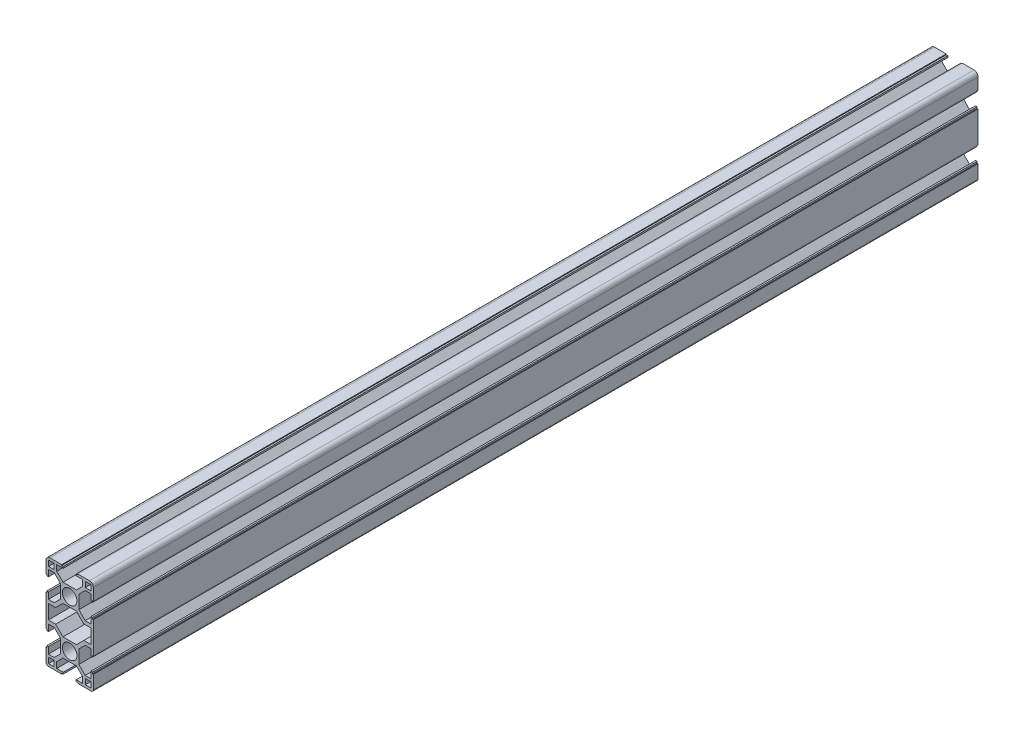
SolidWorks part; units mm, degrees
material "A6061 T6"
ref_plane "前视基准面" through (0, 0, 0) normal (0, 0, 1) x (1, 0, 0)
ref_plane "上视基准面" through (0, 0, 0) normal (0, 1, 0) x (1, 0, 0)
ref_plane "右视基准面" through (0, 0, 0) normal (1, 0, 0) x (0, 0, -1)
sketch "草图1" plane through (0, 0, 0) normal (0, 1, 0) x (1, 0, 0)
  line L0 (0, 0) -> (0, 560)
  dimension "D1" = 560
other "铝型材 30 X 60L X R2.5(1)"
ref_plane "基准面1" through (0, 0, 0) normal (0, 0, -1) x (-1, 0, 0)
sketch "Sketch1" plane through (0, 0, 0) normal (0, 0, -1) x (-1, 0, 0)
  line L0 (-5.1, 15) -> (-5.1, 14.5)
  line L1 (-5.1, 14.5) -> (-4.1, 14.5)
  line L2 (-4.1, 14.5) -> (-4.1, 13.5)
  line L3 (-4.1, 13.5) -> (-8.25, 13.5)
  line L4 (8.9, -10.45) -> (4.25, -5.8)
  line L5 (-15, -24.9) -> (-15, -5.1)
  line L6 (12.5, 15) -> (5.1, 15)
  line L7 (15, 12.5) -> (15, 5.1)
  line L8 (0, 15) -> (0, 0) construction
  line L9 (0, 0) -> (15, 0) construction
  line L10 (-8.25, 13.5) -> (-8.25, 9.8)
  line L11 (-8.25, 9.8) -> (-4.25, 5.8)
  line L12 (-4.25, 5.8) -> (4.25, 5.8)
  line L13 (8.25, 9.8) -> (4.25, 5.8)
  line L14 (8.25, 13.5) -> (8.25, 9.8)
  line L15 (4.1, 13.5) -> (8.25, 13.5)
  line L16 (4.1, 14.5) -> (4.1, 13.5)
  line L17 (5.1, 14.5) -> (4.1, 14.5)
  line L18 (5.1, 15) -> (5.1, 14.5)
  line L19 (-5.1, 15) -> (-12.5, 15)
  line L20 (15, 5.1) -> (14.5, 5.1)
  line L21 (14.5, 5.1) -> (14.5, 4.1)
  line L22 (14.5, 4.1) -> (13.5, 4.1)
  line L23 (13.5, 4.1) -> (13.5, 8.25)
  line L24 (13.5, 8.25) -> (9.8, 8.25)
  line L25 (9.8, 8.25) -> (5.8, 4.25)
  line L26 (5.8, 4.25) -> (5.8, -4.25)
  line L27 (9.8, -8.25) -> (5.8, -4.25)
  line L28 (13.5, -8.25) -> (9.8, -8.25)
  line L29 (13.5, -4.1) -> (13.5, -8.25)
  line L30 (14.5, -4.1) -> (13.5, -4.1)
  line L31 (14.5, -5.1) -> (14.5, -4.1)
  line L32 (15, -5.1) -> (14.5, -5.1)
  line L33 (8.9, -19.55) -> (4.25, -24.2)
  line L34 (-8.9, -19.55) -> (-4.25, -24.2)
  line L35 (-8.9, -10.45) -> (-4.25, -5.8)
  line L36 (-13.5, -10.45) -> (-8.9, -10.45)
  line L37 (-13.5, -19.55) -> (-8.9, -19.55)
  line L38 (-13.5, -10.45) -> (-9.8, -10.45) construction
  line L39 (4.25, -5.8) -> (-4.25, -5.8)
  line L40 (-13.5, -19.55) -> (-9.8, -19.55) construction
  line L41 (-13.5, -10.45) -> (-13.5, -19.55)
  line L42 (13.5, -10.45) -> (13.5, -19.55)
  line L43 (8.9, -10.45) -> (13.5, -10.45)
  line L44 (8.9, -19.55) -> (13.5, -19.55)
  line L45 (-11.625, 11.625) -> (-11.625, 16.245) construction
  line L46 (-15, -5.1) -> (-14.5, -5.1)
  line L47 (-14.5, -5.1) -> (-14.5, -4.1)
  line L48 (-14.5, -4.1) -> (-13.5, -4.1)
  line L49 (-13.5, -4.1) -> (-13.5, -8.25)
  line L50 (-13.5, -8.25) -> (-9.8, -8.25)
  line L51 (-9.8, -8.25) -> (-5.8, -4.25)
  line L52 (-5.8, -4.25) -> (-5.8, 4.25)
  line L53 (-9.8, 8.25) -> (-5.8, 4.25)
  line L54 (-13.5, 8.25) -> (-9.8, 8.25)
  line L55 (-13.5, 4.1) -> (-13.5, 8.25)
  line L56 (-14.5, 4.1) -> (-13.5, 4.1)
  line L57 (-14.5, 5.1) -> (-14.5, 4.1)
  line L58 (-15, 5.1) -> (-14.5, 5.1)
  line L59 (-13.375, 13.375) -> (-9.875, 13.375)
  line L60 (-15, 5.1) -> (-15, 12.5)
  line L61 (15, -5.1) -> (15, -24.9)
  line L62 (-13.375, 13.375) -> (-13.375, 9.875)
  line L63 (-13.375, 9.875) -> (-9.875, 9.875)
  line L64 (-9.875, 13.375) -> (-9.875, 9.875)
  line L65 (-11.625, 11.625) -> (-7.4229, 11.625) construction
  line L66 (-13.5, -45) -> (-5.1, -45)
  line L67 (-15, -43.5) -> (-15, -35.1)
  line L68 (9.875, 13.375) -> (13.375, 13.375)
  line L69 (9.875, 13.375) -> (9.875, 9.875)
  line L70 (9.875, 9.875) -> (13.375, 9.875)
  line L71 (13.375, 13.375) -> (13.375, 9.875)
  line L72 (-4.25, -24.2) -> (4.25, -24.2)
  line L73 (-13.375, -39.875) -> (-9.875, -39.875)
  line L74 (-13.375, -39.875) -> (-13.375, -43.375)
  line L75 (-13.375, -43.375) -> (-9.875, -43.375)
  line L76 (-9.875, -39.875) -> (-9.875, -43.375)
  line L77 (9.875, -39.875) -> (13.375, -39.875)
  line L78 (9.875, -39.875) -> (9.875, -43.375)
  line L79 (9.875, -43.375) -> (13.375, -43.375)
  line L80 (15, -24.9) -> (14.5, -24.9)
  line L81 (14.5, -24.9) -> (14.5, -25.9)
  line L82 (14.5, -25.9) -> (13.5, -25.9)
  line L83 (13.5, -25.9) -> (13.5, -21.75)
  line L84 (13.5, -21.75) -> (9.8, -21.75)
  line L85 (9.8, -21.75) -> (5.8, -25.75)
  line L86 (5.8, -25.75) -> (5.8, -34.25)
  line L87 (9.8, -38.25) -> (5.8, -34.25)
  line L88 (13.5, -38.25) -> (9.8, -38.25)
  line L89 (13.5, -34.1) -> (13.5, -38.25)
  line L90 (14.5, -34.1) -> (13.5, -34.1)
  line L91 (14.5, -35.1) -> (14.5, -34.1)
  line L92 (15, -35.1) -> (14.5, -35.1)
  line L93 (5.1, -45) -> (5.1, -44.5)
  line L94 (5.1, -44.5) -> (4.1, -44.5)
  line L95 (4.1, -44.5) -> (4.1, -43.5)
  line L96 (4.1, -43.5) -> (8.25, -43.5)
  line L97 (8.25, -43.5) -> (8.25, -39.8)
  line L98 (8.25, -39.8) -> (4.25, -35.8)
  line L99 (4.25, -35.8) -> (-4.25, -35.8)
  line L100 (-8.25, -39.8) -> (-4.25, -35.8)
  line L101 (-8.25, -43.5) -> (-8.25, -39.8)
  line L102 (-4.1, -43.5) -> (-8.25, -43.5)
  line L103 (-4.1, -44.5) -> (-4.1, -43.5)
  line L104 (-5.1, -44.5) -> (-4.1, -44.5)
  line L105 (-5.1, -45) -> (-5.1, -44.5)
  line L106 (-15, -35.1) -> (-14.5, -35.1)
  line L107 (-14.5, -35.1) -> (-14.5, -34.1)
  line L108 (-14.5, -34.1) -> (-13.5, -34.1)
  line L109 (-13.5, -34.1) -> (-13.5, -38.25)
  line L110 (-13.5, -38.25) -> (-9.8, -38.25)
  line L111 (-9.8, -38.25) -> (-5.8, -34.25)
  line L112 (-5.8, -34.25) -> (-5.8, -25.75)
  line L113 (-9.8, -21.75) -> (-5.8, -25.75)
  line L114 (-13.5, -21.75) -> (-9.8, -21.75)
  line L115 (-13.5, -25.9) -> (-13.5, -21.75)
  line L116 (-14.5, -25.9) -> (-13.5, -25.9)
  line L117 (-14.5, -24.9) -> (-14.5, -25.9)
  line L118 (-15, -24.9) -> (-14.5, -24.9)
  line L119 (5.1, -45) -> (13.5, -45)
  line L120 (13.375, -39.875) -> (13.375, -43.375)
  line L121 (15, -35.1) -> (15, -43.5)
  line L122 (0, -30) -> (15, -30) construction
  line L125 (5.1, -15) -> (5.1, -14.5) [skipped]
  line L127 (5.1, -14.5) -> (4.1, -14.5) [skipped]
  line L129 (4.1, -14.5) -> (4.1, -13.5) [skipped]
  line L131 (4.1, -13.5) -> (8.25, -13.5) [skipped]
  line L133 (-4.1, -13.5) -> (-8.25, -13.5) [skipped]
  line L135 (-4.1, -14.5) -> (-4.1, -13.5) [skipped]
  line L137 (-5.1, -14.5) -> (-4.1, -14.5) [skipped]
  line L139 (-5.1, -15) -> (-5.1, -14.5) [skipped]
  line L141 (-5.1, -15) -> (-5.1, -15.5) [skipped]
  line L142 (-5.1, -15.5) -> (-4.1, -15.5) [skipped]
  line L143 (-4.1, -15.5) -> (-4.1, -16.5) [skipped]
  line L144 (-4.1, -16.5) -> (-8.25, -16.5) [skipped]
  line L145 (12.5, -15) -> (5.1, -15) [skipped]
  line L146 (4.1, -16.5) -> (8.25, -16.5) [skipped]
  line L147 (4.1, -15.5) -> (4.1, -16.5) [skipped]
  line L148 (5.1, -15.5) -> (4.1, -15.5) [skipped]
  line L149 (5.1, -15) -> (5.1, -15.5) [skipped]
  line L150 (-5.1, -15) -> (-12.5, -15) [skipped]
  line L151 (-15, -24.9) -> (-15, -17.5) [skipped]
  line L152 (15, -17.5) -> (15, -24.9) [skipped]
  line L154 (-8.25, -13.5) -> (-8.25, -9.8) [skipped]
  line L156 (8.25, -13.5) -> (8.25, -9.8) [skipped]
  line L157 (8.25, -16.5) -> (8.25, -20.2) [skipped]
  line L158 (-8.25, -16.5) -> (-8.25, -20.2) [skipped]
  line L160 (-12.5, -14.05) -> (-9.7895, -11.3395) [skipped]
  line L161 (18.444, -10.006) -> (14.8, -13.65) [skipped]
  line L163 (11.9857, -13.5357) -> (9.7894, -11.3394) [skipped]
  line L164 (-15.9344, -12.5156) -> (-14.8, -13.65) [skipped]
  line L165 (9.7894, -15) -> (-9.8, -15) construction
  circle A0 centre (0, 0) radius 4.6
  arc A1 (-15, 12.5) -> (-12.5, 15) centre (-12.5, 12.5) cw
  arc A2 (15, 12.5) -> (12.5, 15) centre (12.5, 12.5) ccw
  arc A3 (15, -43.5) -> (13.5, -45) centre (13.5, -43.5) cw
  arc A4 (-15, -43.5) -> (-13.5, -45) centre (-13.5, -43.5) ccw
  circle A5 centre (0, -30) radius 4.6
  arc A12 (-15, -17.5) -> (-12.5, -15) centre (-12.5, -17.5) cw [skipped]
  arc A13 (15, -17.5) -> (12.5, -15) centre (12.5, -17.5) ccw [skipped]
  point P0 (-10, 0)
  point P1 (10, 0)
  point P2 (0, 20)
  point P4 (0, 0)
  point P5 (0, 0)
  point P6 (-10, 0)
  point P7 (15, 15)
  point P8 (-15, 15)
  point P12 (-15, -15)
  point P13 (15, -15)
  point P15 (0, -10)
  point P16 (10, 0)
  point P36 (-15, 15)
  point P39 (15, 15)
  point P43 (-10, -30)
  point P44 (10, -30)
  point P88 (0, -30)
  point P89 (0, -30)
  point P90 (-10, -30)
  point P91 (10, -30)
  point P102 (15, -45)
  point P120 (-15, -45)
  point P121 (0, 0)
  dimension "D1" = 16.5
  dimension "D2" = 30
  dimension "D3" = 8.2
  dimension "D4" = 10.2
  dimension "D5" = 9.2
  dimension "D6" = 9.2
  dimension "D7" = 2.5
  dimension "D8" = 45
  dimension "D14" = 30
  dimension "D15" = 1.5
  dimension "D9" = 0.5
  dimension "D10" = 1
  dimension "D11" = 8.5
  dimension "D12" = 15
  dimension "D13" = 60
  dimension "D16" = 45
  dimension "D17" = 45
  dimension "D18" = 10.2
  dimension "D19" = 8.2
  dimension "D20" = 2.2
  dimension "D22" = 3.5
  dimension "D21" = 2.2
hole_wizard "打孔尺寸(%根据)内六角圆柱头螺钉的类型1" positions "草图3" profile "草图4" counterbore size "M6" standard "GB" end condition through all
sketch "草图3" plane through (-15, 0, 0) normal (-1, 0, 0) x (0, 0, 1)
  line L0 (-560, 5.1) -> (-560, 12.5) construction
  line L1 (-560, 15) -> (0, 15) construction
  line L2 (-560, -45) -> (0, -45) construction
  line L3 (-560, -4.25) -> (-560, 4.25) construction
  point P0 (-550, 0)
  point P2 (-487.5, 0)
  point P4 (-487.5, -30)
  point P6 (-550, -30)
  point P8 (-520, -30)
  point P10 (-520, 0)
  dimension "D1" = 72.5
  dimension "D2" = 15
  dimension "D3" = 15
  dimension "D4" = 10
  dimension "D5" = 30
sketch "草图4" plane through (-15, 0, -550) normal (0, 1, 0) x (0, 0, 1)
  line L0 (0, 0) -> (0, 30)
  line L1 (0, 30) -> (3.3, 30)
  line L3 (3.3, 30) -> (3.3, 6.8)
  line L4 (3.3, 6.8) -> (5.5, 6.8)
  line L5 (5.5, 6.8) -> (5.5, 0)
  line L7 (5.5, 0) -> (0, 0)
  line L11 (0, -6.35) -> (0, 107.95) construction
  dimension "通孔孔直径" = 6.6
  dimension "通孔孔深度" = 30
  dimension "柱形沉头孔直径" = 11
  dimension "柱形沉头孔深度" = 6.8
